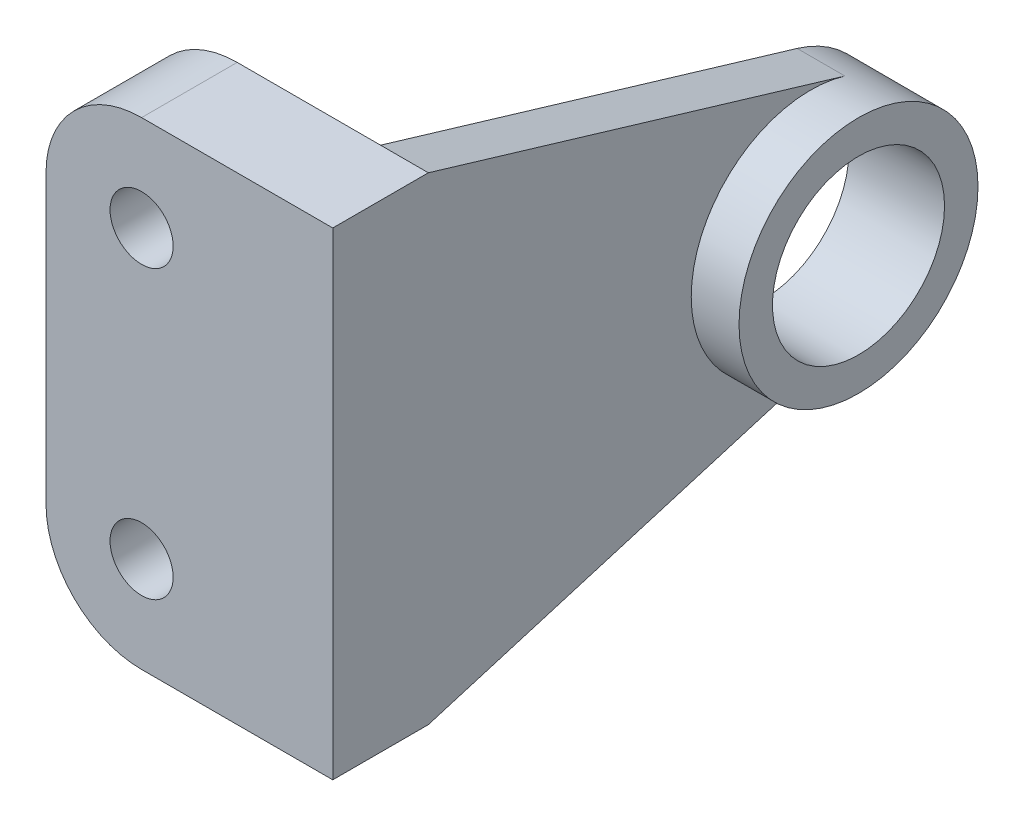
from build123d import *
from build123d.topology import SkipClean

# Parameters (mm, degrees)
SKETCH1_W                                    = 30
SKETCH1_H                                    = 50
BOSS_EXTRUDE1_DEPTH                          = 10
SKETCH2_R                                    = 9
BOSS_EXTRUDE3_DEPTH                          = 5
BOSS_EXTRUDE4_START                          = 5
SKETCH3_R                                    = 12.5
SKETCH3_R_2                                  = 9
BOSS_EXTRUDE4_DEPTH                          = 5
FILLET1_R                                    = 10
CBORE_FOR_M6_HEXAGON_SOCKET_HEAD_CAP_2_COUNT = 2
CBORE_FOR_M6_HEXAGON_SOCKET_HEAD_CAP_2_PITCH = 30
CUT_EXTRUDE1_DEPTH                           = 27
CUT_EXTRUDE1_DEPTH_BACK                      = 19
SKETCH8_R                                    = 3.3


with BuildPart() as part:
    # Sketch1 → Boss-Extrude1 (new body)
    with BuildSketch(Plane.XY):
        Rectangle(SKETCH1_W, SKETCH1_H)
    extrude(amount=BOSS_EXTRUDE1_DEPTH)

    # Sketch2 → Boss-Extrude3 (add)
    with BuildSketch(Plane(origin=(15, -15, 0), x_dir=(0, 1, 0), z_dir=(-1, 0, 0))):
        with BuildLine():
            Line((3.023367754, 43.579145154), (-10, 0))
            Line((-10, 0), (40, 0))
            Line((40, 0), (26.976632246, 43.579145154))
            ThreePointArc((26.976632246, 43.579145154), (15, 52.5), (3.023367754, 43.579145154))
        make_face()
        with Locations(Location((15, 40, 0), (0, 0, 270))):
            Circle(SKETCH2_R, mode=Mode.SUBTRACT)
    extrude(amount=BOSS_EXTRUDE3_DEPTH)

    # Sketch3 → Boss-Extrude4 (add)
    with SkipClean():  # the faces are left unmerged after this step: merging them gives an invalid solid
        with BuildSketch(Plane(origin=(15, 0, 0), x_dir=(0, 0, -1), z_dir=(1, 0, 0)).offset(BOSS_EXTRUDE4_START)):
            with Locations((40, 0)):
                Circle(SKETCH3_R)
            with Locations((40, 0)):
                Circle(SKETCH3_R_2, mode=Mode.SUBTRACT)
        extrude(amount=-BOSS_EXTRUDE4_DEPTH)

    # Fillet1
    fillet1_edges = [part.edges().sort_by_distance(p)[0] for p in [
        (-15, -25, 5),
        (-15, 25, 5),
    ]]
    fillet(fillet1_edges, radius=FILLET1_R)

    # Sketch4 → CBORE for M6 Hexagon socket head cap screws1 (revolve, cut)
    with BuildSketch(Plane(origin=(-5, -15, 0), x_dir=(0, 1, 0), z_dir=(1, 0, 0))):
        Polygon((0, 0), (0, 5), (3.3, 3.017159957), (3.3, 5), (5.5, 5), (5.5, 0), align=None)
    cbore_for_m6_hexagon_socket_head_cap_scr = revolve(axis=Axis((-5, -15, -6.35), (0, 0, 1)), mode=Mode.SUBTRACT)

    # CBORE for M6 Hexagon socket head cap 2: CBORE for M6 Hexagon socket head cap screws1 ×2
    with Locations(*[(0, i * CBORE_FOR_M6_HEXAGON_SOCKET_HEAD_CAP_2_PITCH, 0) for i in range(1, CBORE_FOR_M6_HEXAGON_SOCKET_HEAD_CAP_2_COUNT)]):
        add(cbore_for_m6_hexagon_socket_head_cap_scr, mode=Mode.SUBTRACT)

    # Sketch8 → Cut-Extrude1 (cut, two sides: drawn at the far end of the back side and taken through both)
    with BuildSketch(Plane(origin=(0, 0, 5), x_dir=(-1, 0, 0), z_dir=(0, 0, -1)).offset(-CUT_EXTRUDE1_DEPTH_BACK)):
        with Locations(Location((5, -15, 0), (0, 0, 180))):
            Circle(SKETCH8_R)
        with Locations(Location((5, 15, 0), (0, 0, 180))):
            Circle(SKETCH8_R)
    extrude(amount=CUT_EXTRUDE1_DEPTH + CUT_EXTRUDE1_DEPTH_BACK, mode=Mode.SUBTRACT)


solid = part.part
